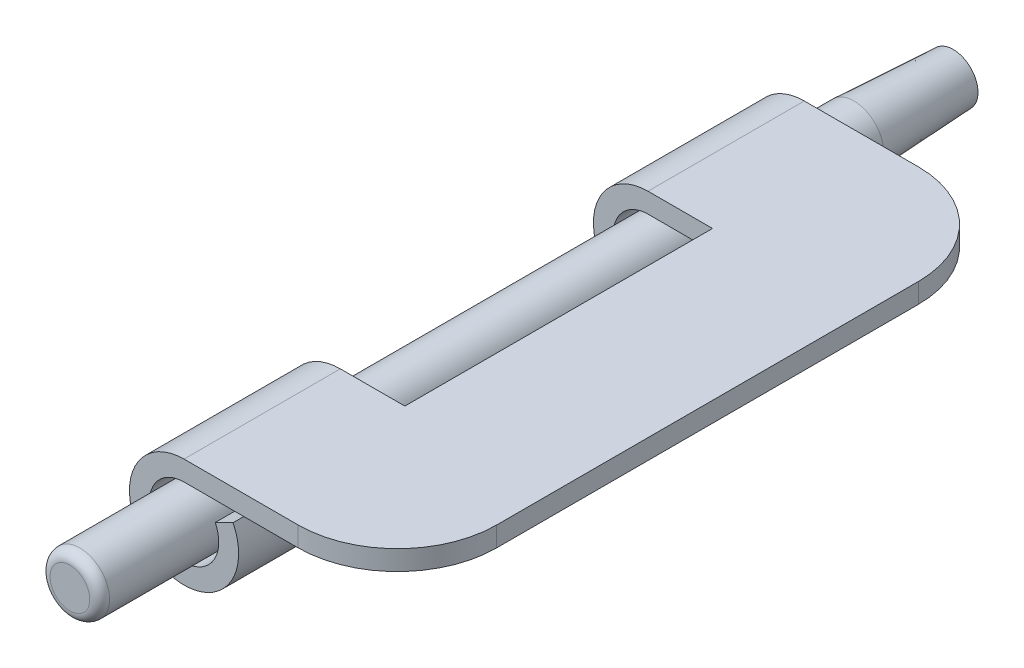
SolidWorks part; units mm, degrees
material "碳钢镀锌"
ref_plane "前视" through (0, 0, 0) normal (0, 0, 1) x (1, 0, 0)
ref_plane "上视" through (0, 0, 0) normal (0, 1, 0) x (1, 0, 0)
ref_plane "右视" through (0, 0, 0) normal (1, 0, 0) x (0, 0, -1)
sketch "草图3" plane through (0, 0, 0) normal (0, 0, 1) x (1, 0, 0)
  line L0 (21.5, 0) -> (0, 0)
  arc A0 (0, 0) -> (3.143, -1.96) centre (0, -3.5) ccw
  dimension "D2" = 7
  dimension "D1" = 21.5
extrude "拉伸-薄壁5" add sketch "草图3" along normal mid plane 62.5 thin contours L0 A0
sketch "草图4" plane through (0, 2, 0) normal (0, 1, 0) x (1, 0, 0)
  line L0 (-5.5, 31.25) -> (-5.5, -31.25) construction
  line L1 (-5.5, 15.5) -> (6.5, 15.5)
  line L2 (-5.5, 15.5) -> (-5.5, -15.5)
  line L3 (-5.5, -15.5) -> (6.5, -15.5)
  line L4 (6.5, 15.5) -> (6.5, -15.5)
  line L5 (21.5, 0) -> (-5.5, 0) construction
  line L6 (21.5, -31.25) -> (21.5, 31.25) construction
  dimension "D1" = 31
  dimension "D2" = 12
extrude "切除-拉伸1" cut sketch "草图4" against normal through all
ref_plane "基准面1" through (0, 0, 42.75) normal (0, 0, 1) x (1, 0, 0)
sketch "草图6" plane through (0, 0, 42.75) normal (0, 0, 1) x (1, 0, 0)
  circle A0 centre (0, -3.5) radius 3
  dimension "D1" = 6
extrude "凸台-拉伸3" add sketch "草图6" against normal blind 89 contours A0
chamfer "倒角1" distance 0.5 distance2 10 1 edges at (3, -3.5, -46.25)
fillet "圆角1" radius 10 2 edges at (21.5, 1, 31.25) (21.5, 1, -31.25)
fillet "圆角2" radius 1 1 edges at (3, -3.5, 42.75)
